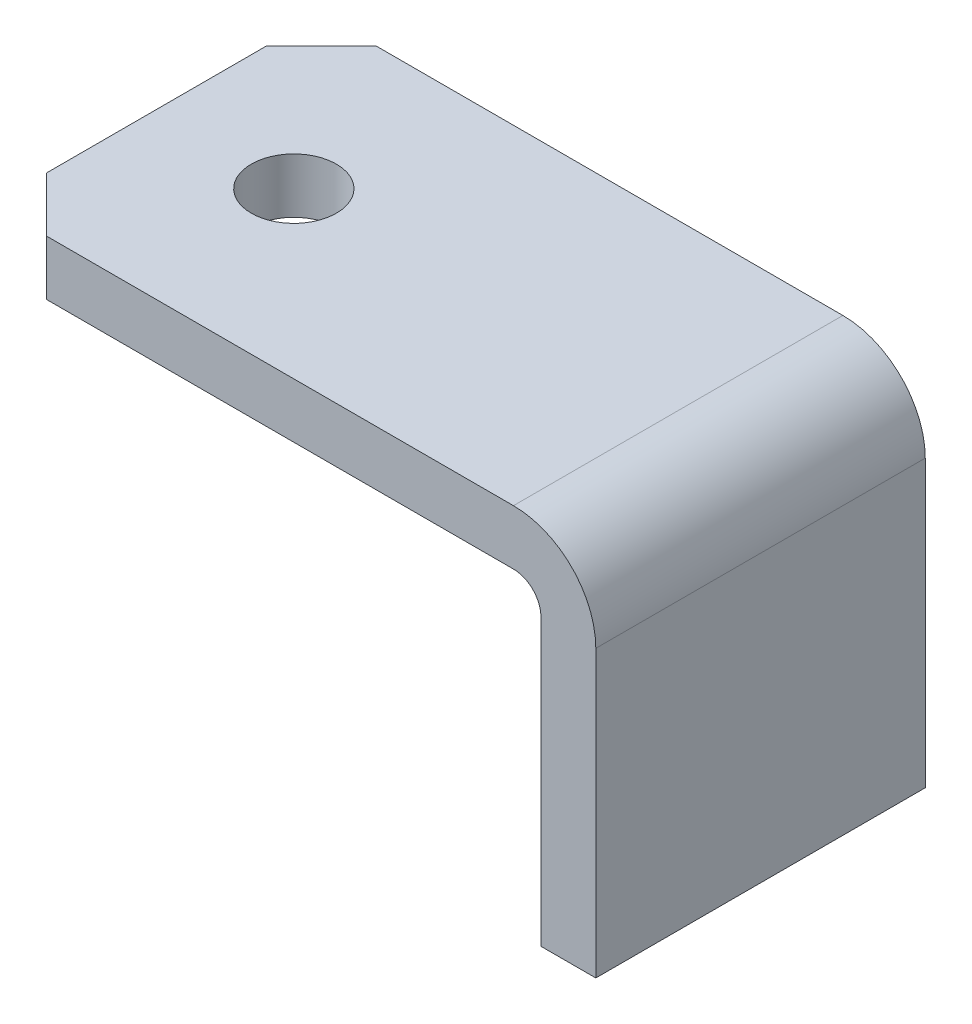
from build123d import *

# Parameters (mm, degrees)
BOSS_EXTRUDE1_DEPTH    = 60
CHAMFER1_SIZE          = 10
M18_TAPPED_HOLE1_D     = 15.5
M18_TAPPED_HOLE1_DEPTH = 43.5
M18_TAPPED_HOLE1_TIP   = 4.656669797


with BuildPart() as part:
    # Sketch1 → Boss-Extrude1 (new body)
    with BuildSketch(Plane.XY):
        with BuildLine():
            Line((0, 0), (95, 0))
            ThreePointArc((95, 0), (105.606601718, -4.393398282), (110, -15))
            Line((110, -15), (110, -67))
            Line((110, -67), (100, -67))
            Line((100, -67), (100, -15))
            ThreePointArc((100, -15), (98.535533906, -11.464466094), (95, -10))
            Line((95, -10), (0, -10))
            Line((0, -10), (0, 0))
        make_face()
    extrude(amount=BOSS_EXTRUDE1_DEPTH)

    # Chamfer1
    chamfer1_edges = [part.edges().sort_by_distance(p)[0] for p in [
        (0, -5, 0),
        (0, -5, 60),
    ]]
    chamfer(chamfer1_edges, length=CHAMFER1_SIZE)

    # M18 Tapped Hole1
    with Locations(Plane(origin=(0, 0, 0), x_dir=(1, 0, 0), z_dir=(0, 1, 0))):
        with Locations((25, -30)):
            Hole(M18_TAPPED_HOLE1_D / 2, depth=M18_TAPPED_HOLE1_DEPTH)
            with Locations((0, 0, -(M18_TAPPED_HOLE1_DEPTH + M18_TAPPED_HOLE1_TIP / 2))):  # 118° drill point
                Cone(0, M18_TAPPED_HOLE1_D / 2, M18_TAPPED_HOLE1_TIP, mode=Mode.SUBTRACT)


solid = part.part
